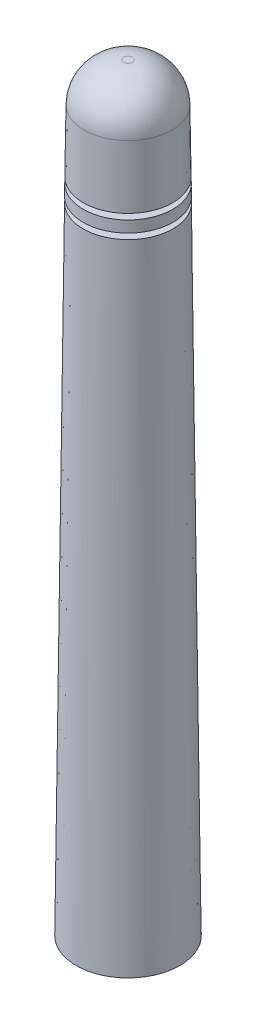
from build123d import *

# Parameters (mm, degrees)
EXTRUDE_1_REACH = 69.614
SKETCH_2_W      = 0.974227423
SKETCH_2_H      = 0.5


with BuildPart() as part:
    # 草图1 → 旋转1 (revolve)
    with BuildSketch(Plane.XY, mode=Mode.PRIVATE) as revolve_1_sk:
        with BuildLine():
            Line((-4.6, 0), (-4, 0))
            Line((-4, 0), (-4, 1))
            Line((-4, 1), (-3.5, 1))
            Line((-3.5, 1), (-3.5, 2.5))
            Line((-3.5, 2.5), (-4, 2.5))
            Line((-4, 2.5), (-4, 4.3))
            Line((-4, 4.3), (-3.5, 4.3))
            Line((-3.5, 4.3), (-3.5, 5.8))
            Line((-3.5, 5.8), (-4, 5.8))
            Line((-4, 5.8), (-4, 7.3))
            Line((-4, 7.3), (-3.5, 7.3))
            Line((-3.5, 7.3), (-3.5, 9.1))
            Line((-3.5, 9.1), (-4, 9.1))
            Line((-4, 9.1), (-4, 10))
            Line((-4, 10), (-2.75, 10))
            Line((-2.75, 10), (-2.575500592, 64.3))
            ThreePointArc((-2.575500592, 64.3), (-2.282607373, 65.007106781), (-1.575500592, 65.3))
            Line((-1.575500592, 65.3), (0, 65.3))
            Line((0, 65.3), (0, 67.3))
            Line((0, 67.3), (-0.391399138, 67.3))
            ThreePointArc((-0.391399138, 67.3), (-2.852382856, 66.288686228), (-3.891179873, 63.839176651))
            Line((-3.891179873, 63.839176651), (-3.969072705, 58.3))
            Line((-3.969072705, 58.3), (-3.25, 58.3))
            Line((-3.25, 58.3), (-3.25, 57.8))
            Line((-3.25, 57.8), (-3.974609916, 57.8))
            Line((-3.974609916, 57.8), (-3.985684336, 56.8))
            Line((-3.985684336, 56.8), (-3.25, 56.8))
            Line((-3.25, 56.8), (-3.25, 56.3))
            Line((-3.25, 56.3), (-3.985684336, 56.3))
            Line((-3.985684336, 56.3), (-4.6, 0))
        make_face()
    revolve(revolve_1_sk.sketch.rotate(Axis((0, 0, 0), (0, 1, 0)), 270), axis=Axis((0, 0, 0), (0, 1, 0)))

    # 凸台-拉伸1: up to this face of the body (flat: up to its plane)
    extrude_1_end = Plane(part.part.faces().sort_by_distance((0, 7.3, 3.886862915))[0])
    # 草图2 → 凸台-拉伸1 (add, up to the picked face)
    with BuildSketch(Plane.XZ, mode=Mode.PRIVATE) as extrude_1_sk1:
        with Locations((-3.887113712, 0)):
            Rectangle(SKETCH_2_W, SKETCH_2_H)
    extrude_1_tool1 = split(extrude(extrude_1_sk1.sketch, amount=-EXTRUDE_1_REACH, mode=Mode.PRIVATE), bisect_by=extrude_1_end, keep=Keep.BOTH, mode=Mode.PRIVATE)
    # 草图2 → 凸台-拉伸1 (add, up to the picked face)
    with BuildSketch(Plane.XZ, mode=Mode.PRIVATE) as extrude_1_sk2:
        with Locations((3.887113712, 0)):
            Rectangle(SKETCH_2_W, SKETCH_2_H)
    extrude_1_tool2 = split(extrude(extrude_1_sk2.sketch, amount=-EXTRUDE_1_REACH, mode=Mode.PRIVATE), bisect_by=extrude_1_end, keep=Keep.BOTH, mode=Mode.PRIVATE)
    add(extrude_1_tool1.solids().sort_by(Axis((-3.887114, 0, 0), (0, 1, 0)))[0])
    add(extrude_1_tool2.solids().sort_by(Axis((3.887114, 0, 0), (0, 1, 0)))[0])


solid = part.part
